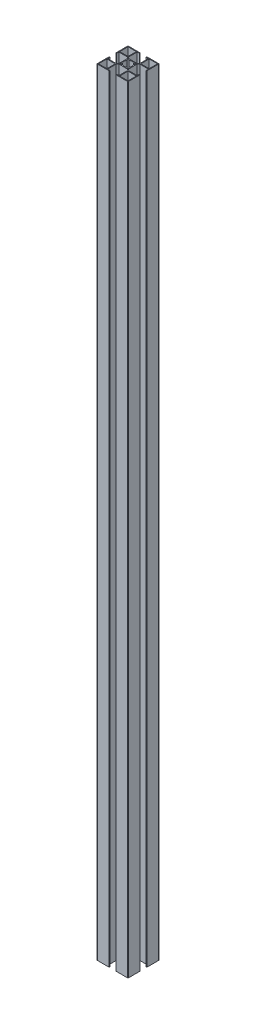
from build123d import *

# Parameters (mm, degrees)
SKETCH1_W               = 10.85
SKETCH1_H               = 10.85
BOSS_EXTRUDE1_DEPTH     = 1000
MIRROR2_COPY_1_SKETCH_W = 10.85
MIRROR2_COPY_1_SKETCH_H = 10.85
MIRROR2_COPY_1_DEPTH    = 1000


with BuildPart() as part:
    # Sketch1 → Boss-Extrude1 (new body)
    with BuildSketch(Plane(origin=(0, 0, 0), x_dir=(1, 0, 0), z_dir=(0, 1, 0))):
        with BuildLine():
            Line((-4.3, 20), (-19.5, 20))
            ThreePointArc((-19.5, 20), (-19.853553391, 19.853553391), (-20, 19.5))
            Line((-20, 19.5), (-20, 4.3))
            Line((-20, 4.3), (-19.05, 4.3))
            Line((-19.05, 4.3), (-19.05, 7.25))
            Line((-19.05, 7.25), (-7.921751442, 7.25))
            Line((-7.921751442, 7.25), (-6.2, 5.528248558))
            Line((-6.2, 5.528248558), (-6.2, 0))
            Line((-6.2, 0), (-5.3, 0))
            ThreePointArc((-5.3, 0), (-5.066731596, 1.555066215), (-4.387460025, 2.973246463))
            Line((-4.387460025, 2.973246463), (-5.091168825, 3.676955262))
            ThreePointArc((-5.091168825, 3.676955262), (-5.091168825, 5.091168825), (-3.676955262, 5.091168825))
            Line((-3.676955262, 5.091168825), (-2.973246463, 4.387460025))
            ThreePointArc((-2.973246463, 4.387460025), (-1.555066215, 5.066731596), (0, 5.3))
            Line((0, 5.3), (0, 6.2))
            Line((0, 6.2), (-5.528248558, 6.2))
            Line((-5.528248558, 6.2), (-7.25, 7.921751442))
            Line((-7.25, 7.921751442), (-7.25, 19.05))
            Line((-7.25, 19.05), (-4.3, 19.05))
            Line((-4.3, 19.05), (-4.3, 20))
        make_face()
        with Locations((-13.625, 13.625)):
            Rectangle(SKETCH1_W, SKETCH1_H, mode=Mode.SUBTRACT)
    boss_extrude1 = extrude(amount=BOSS_EXTRUDE1_DEPTH)

    # Mirror1: Boss-Extrude1 across plane
    add(boss_extrude1.mirror(Plane(origin=(0, 0, 0), x_dir=(0, 0, 1), z_dir=(1, 0, 0))))

    # Mirror2: Boss-Extrude1 across plane
    add(boss_extrude1.mirror(Plane.XY))

    # Mirror2 copy 1 sketch → Mirror2 copy 1 (add)
    with BuildSketch(Plane(origin=(0, 0, 0), x_dir=(-1, 0, 0), z_dir=(0, 1, 0))):
        with BuildLine():
            Line((-4.3, 20), (-19.5, 20))
            ThreePointArc((-19.5, 20), (-19.853553391, 19.853553391), (-20, 19.5))
            Line((-20, 19.5), (-20, 4.3))
            Line((-20, 4.3), (-19.05, 4.3))
            Line((-19.05, 4.3), (-19.05, 7.25))
            Line((-19.05, 7.25), (-7.921751442, 7.25))
            Line((-7.921751442, 7.25), (-6.2, 5.528248558))
            Line((-6.2, 5.528248558), (-6.2, 0))
            Line((-6.2, 0), (-5.3, 0))
            ThreePointArc((-5.3, 0), (-5.066731596, 1.555066215), (-4.387460025, 2.973246463))
            Line((-4.387460025, 2.973246463), (-5.091168825, 3.676955262))
            ThreePointArc((-5.091168825, 3.676955262), (-5.091168825, 5.091168825), (-3.676955262, 5.091168825))
            Line((-3.676955262, 5.091168825), (-2.973246463, 4.387460025))
            ThreePointArc((-2.973246463, 4.387460025), (-1.555066215, 5.066731596), (0, 5.3))
            Line((0, 5.3), (0, 6.2))
            Line((0, 6.2), (-5.528248558, 6.2))
            Line((-5.528248558, 6.2), (-7.25, 7.921751442))
            Line((-7.25, 7.921751442), (-7.25, 19.05))
            Line((-7.25, 19.05), (-4.3, 19.05))
            Line((-4.3, 19.05), (-4.3, 20))
        make_face()
        with Locations((-13.625, 13.625)):
            Rectangle(MIRROR2_COPY_1_SKETCH_W, MIRROR2_COPY_1_SKETCH_H, mode=Mode.SUBTRACT)
    extrude(amount=MIRROR2_COPY_1_DEPTH)


solid = part.part
